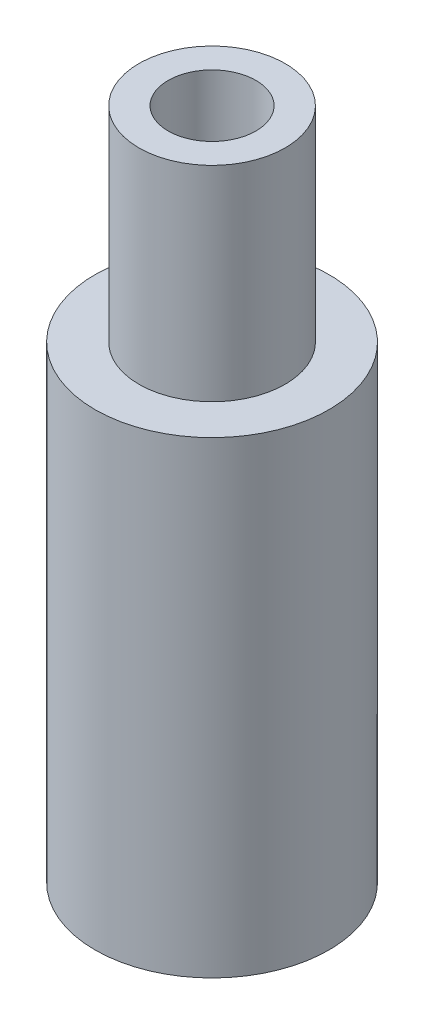
SolidWorks part; units mm, degrees
material "普通碳钢"
ref_plane "Front Plane" through (0, 0, 0) normal (0, 0, 1) x (1, 0, 0)
ref_plane "Top Plane" through (0, 0, 0) normal (0, 1, 0) x (1, 0, 0)
ref_plane "Right Plane" through (0, 0, 0) normal (1, 0, 0) x (0, 0, -1)
sketch "Sketch1" plane through (0, 0, 0) normal (0, 0, 1) x (1, 0, 0)
  line L0 (-73.1294, -60) -> (-73.1294, -175.0657) construction
  line L2 (-65.6294, -27.9727) -> (-60.6294, -27.9727)
  line L3 (-60.6294, -27.9727) -> (-60.6294, -62.9727)
  line L4 (-60.6294, -62.9727) -> (-53.1294, -62.9727)
  line L5 (-53.1294, -62.9727) -> (-53.1294, -142.9727)
  line L6 (-53.1294, -142.9727) -> (-73.1294, -142.9727)
  line L7 (-73.1294, -142.9727) -> (-73.1294, -137.9727)
  line L8 (-73.1294, -137.9727) -> (-58.1294, -137.9727)
  line L9 (-58.1294, -137.9727) -> (-58.1294, -67.9727)
  line L10 (-58.1294, -67.9727) -> (-65.6294, -67.9727)
  line L11 (-65.6294, -27.9727) -> (-65.6294, -67.9727)
  dimension "D1" = 5
  dimension "D2" = 5
  dimension "D3" = 5
  dimension "D4" = 5
  dimension "D5" = 20
  dimension "D6" = 7.5
  dimension "D7" = 35
  dimension "D8" = 80
revolve "Revolve1" add sketch "Sketch1" angle 360 about L0
